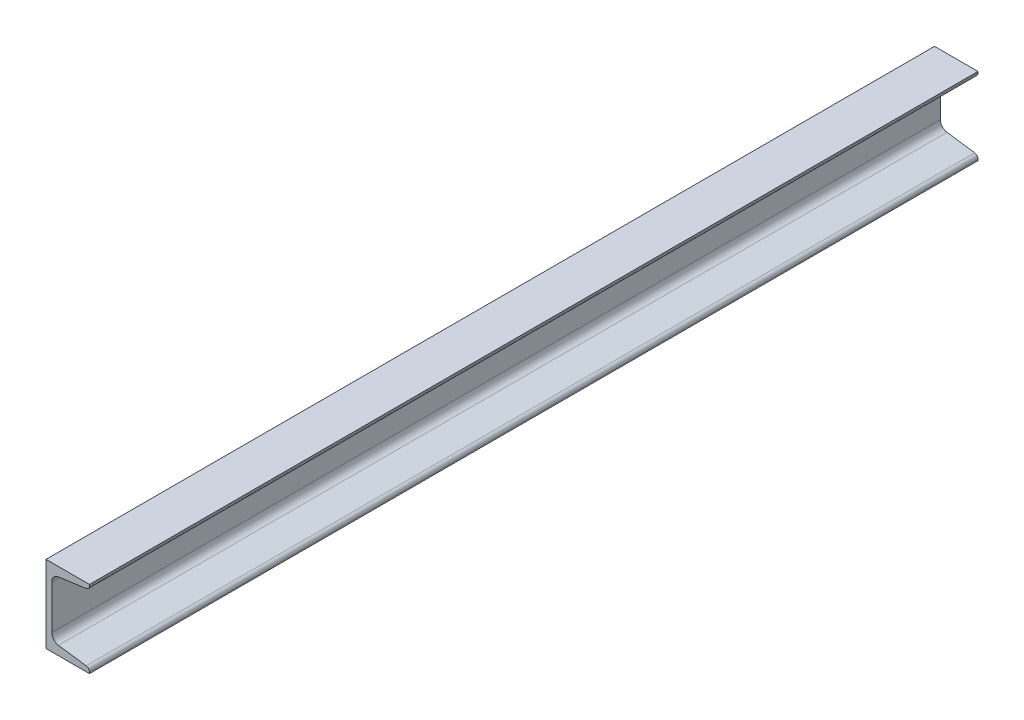
from build123d import *

# Parameters (mm, degrees)
BOSS_EXTRUDE1_DEPTH = 920


with BuildPart() as part:
    # Sketch1 → Boss-Extrude1 (new body)
    with BuildSketch(Plane.XY):
        with BuildLine():
            Line((0, 0), (-45, 0))
            Line((-45, 0), (-45, -80))
            Line((-45, -80), (0, -80))
            Line((0, -80), (0, -78.639315732))
            ThreePointArc((0, -78.639315732), (-0.981161679, -76.015079616), (-3.443307596, -74.678243457))
            Line((-3.443307596, -74.678243457), (-32.113384808, -70.648926875))
            ThreePointArc((-32.113384808, -70.648926875), (-37.037676642, -67.975254557), (-39, -62.726782325))
            Line((-39, -62.726782325), (-39, -17.273217675))
            ThreePointArc((-39, -17.273217675), (-37.037676642, -12.024745443), (-32.113384808, -9.351073125))
            Line((-32.113384808, -9.351073125), (-3.443307596, -5.321756543))
            ThreePointArc((-3.443307596, -5.321756543), (-0.981161679, -3.984920384), (0, -1.360684268))
            Line((0, -1.360684268), (0, 0))
        make_face()
    extrude(amount=BOSS_EXTRUDE1_DEPTH)


solid = part.part
